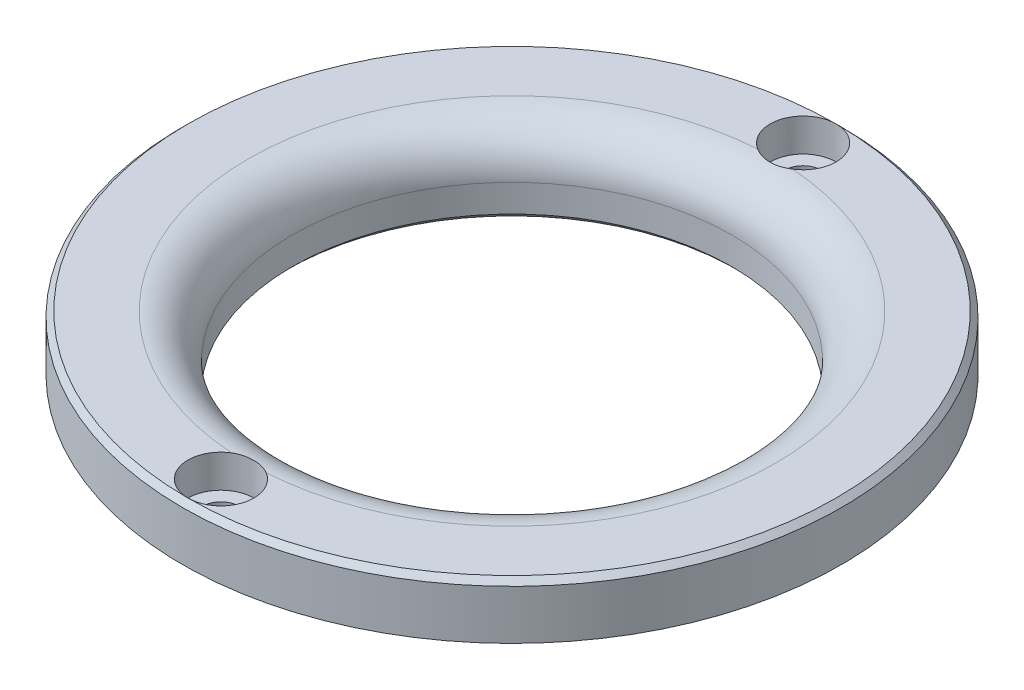
SolidWorks part; units mm, degrees
ref_plane "Front Plane" through (0, 0, 0) normal (0, 0, 1) x (1, 0, 0)
ref_plane "Top Plane" through (0, 0, 0) normal (0, 1, 0) x (1, 0, 0)
ref_plane "Right Plane" through (0, 0, 0) normal (1, 0, 0) x (0, 0, -1)
sketch "Sketch1" plane through (0, 0, 0) normal (0, 1, 0) x (1, 0, 0)
  circle A0 centre (0, 0) radius 20
  circle A1 centre (0, 0) radius 30
  dimension "D1" = 40
  dimension "D2" = 60
extrude "Boss-Extrude1" add sketch "Sketch1" along normal mid plane 7
sketch "Sketch2" plane through (0, -3.5, 0) normal (0, -1, 0) x (1, 0, 0)
  circle A0 centre (0, 0) radius 23
  dimension "D1" = 46
extrude "Cut-Extrude1" cut sketch "Sketch2" against normal blind 2 flip side to cut
fillet "Fillet1" radius 4 1 edges at (0, 3.5, 20)
chamfer "Chamfer1" distance 0.5 angle 45 3 edges at (0, -3.5, -23) (0, -3.5, 20) (0, 3.5, 30)
hole_wizard "Hole Size by Socket Head Cap Screw Type1" positions "Sketch4" profile "Sketch3" counterbore size "M3" standard "Gb" end condition through all
sketch "Sketch4" plane through (0, 3.5, 0) normal (0, 1, 0) x (1, 0, 0)
  line L0 (0, 0) -> (42.9503, 0) construction
  point P0 (0, -26.5)
  point P2 (0, 26.5)
  dimension "D1" = 53
sketch "Sketch3" plane through (0, 3.5, 26.5) normal (1, 0, 0) x (0, 0, 1)
  line L0 (0, 0) -> (0, 7)
  line L1 (0, 7) -> (1.7, 7)
  line L3 (1.7, 7) -> (1.7, 3)
  line L4 (1.7, 3) -> (3, 3)
  line L5 (3, 3) -> (3, 0)
  line L7 (3, 0) -> (0, 0)
  line L11 (0, -6.35) -> (0, 107.95) construction
  dimension "通孔孔直径" = 3.4
  dimension "通孔孔深度" = 7
  dimension "柱形沉头孔直径" = 6
  dimension "柱形沉头孔深度" = 3
